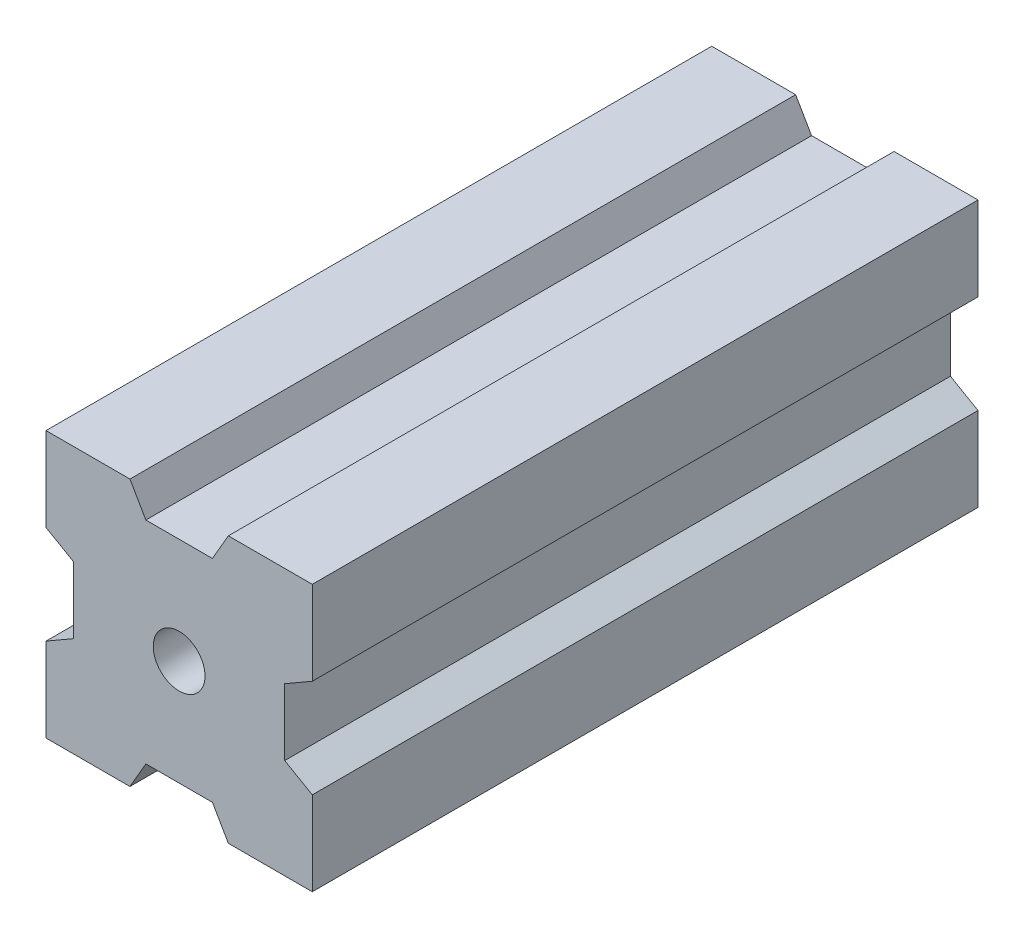
SolidWorks part; units mm, degrees
ref_plane "前视基准面" through (0, 0, 0) normal (0, 0, 1) x (1, 0, 0)
ref_plane "上视基准面" through (0, 0, 0) normal (0, 1, 0) x (1, 0, 0)
ref_plane "右视基准面" through (0, 0, 0) normal (1, 0, 0) x (0, 0, -1)
sketch "草图1" plane through (0, 0, 0) normal (0, 0, 1) x (1, 0, 0)
  line L1 (10, -10) -> (-10, -10)
  line L2 (10, -10) -> (10, 10)
  line L3 (10, 10) -> (-10, 10)
  line L4 (-10, -10) -> (-10, 10)
  line L5 (10, -10) -> (-10, 10) construction
  line L6 (10, 10) -> (-10, -10) construction
  circle A0 centre (0, 0) radius 1.9444
  point P0 (0, 0)
  dimension "D1" = 20
extrude "凸台-拉伸1" add sketch "草图1" along normal mid plane 50
sketch "草图2" plane through (0, 0, 25) normal (0, 0, 1) x (1, 0, 0)
  line L0 (-3.6944, 10) -> (-2.5, 7.9312)
  line L1 (10, 10) -> (-10, 10) construction
  line L2 (-2.5, 7.9312) -> (2.5, 7.9312)
  line L3 (2.5, 7.9312) -> (3.6944, 10)
  line L4 (0, 10) -> (0, 7.9312) construction
  line L5 (-3.6944, 10) -> (3.6944, 10) construction
  dimension "D1" = 5
  dimension "D2" = 60
extrude "切除-拉伸1" cut sketch "草图2" against normal through all and the other way through all
pattern_circular "阵列(圆周)1" count 4 over 360 about axis through (0, 0, 25) along (0, 0, -1) of "切除-拉伸1"
